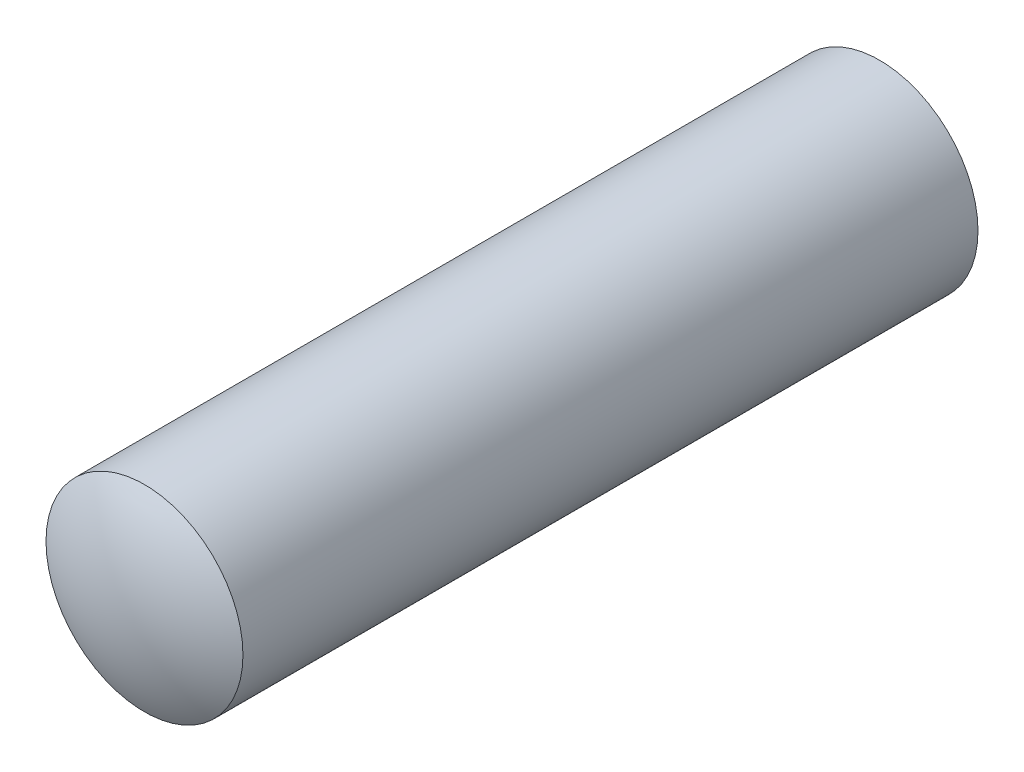
SolidWorks part; units mm, degrees
ref_plane "Front" through (0, 0, 0) normal (0, 0, 1) x (1, 0, 0)
ref_plane "Top" through (0, 0, 0) normal (0, 1, 0) x (1, 0, 0)
ref_plane "Right" through (0, 0, 0) normal (1, 0, 0) x (0, 0, -1)
sketch "Logo3_Revol_Axis" plane through (0, 0, 0) normal (0, 1, 0) x (1, 0, 0)
  line L0 (0, -30.1653) -> (0, 30.1653) construction
sketch "Logo3_bib1" plane through (0, 0, 0) normal (0, -1, 0) x (-1, 0, 0)
  line L0 (0, 8) -> (0, -8)
  line L1 (2, 7.4641) -> (2, -7.4641)
  line L10 (0, 47.5372) -> (0, -34.1764) construction
  arc A0 (2, 7.4641) -> (0, 8) centre (0, 4) ccw
  arc A1 (0, -8) -> (2, -7.4641) centre (0, -4) ccw
revolve "Revolve1" add sketch "Logo3_bib1" angle 360 about L10
equation "\"ray2@XZQB7_bib1\" = \"XZQB7_d1@XZQB7_bib1\""
equation "\"Ray1@XZQB7_bib1\" = \"XZQB7_d1@XZQB7_bib1\""
equation "\"dia1@XZQB7_bib1\" = \"XZQB7_d1@XZQB7_bib1\"/2"
